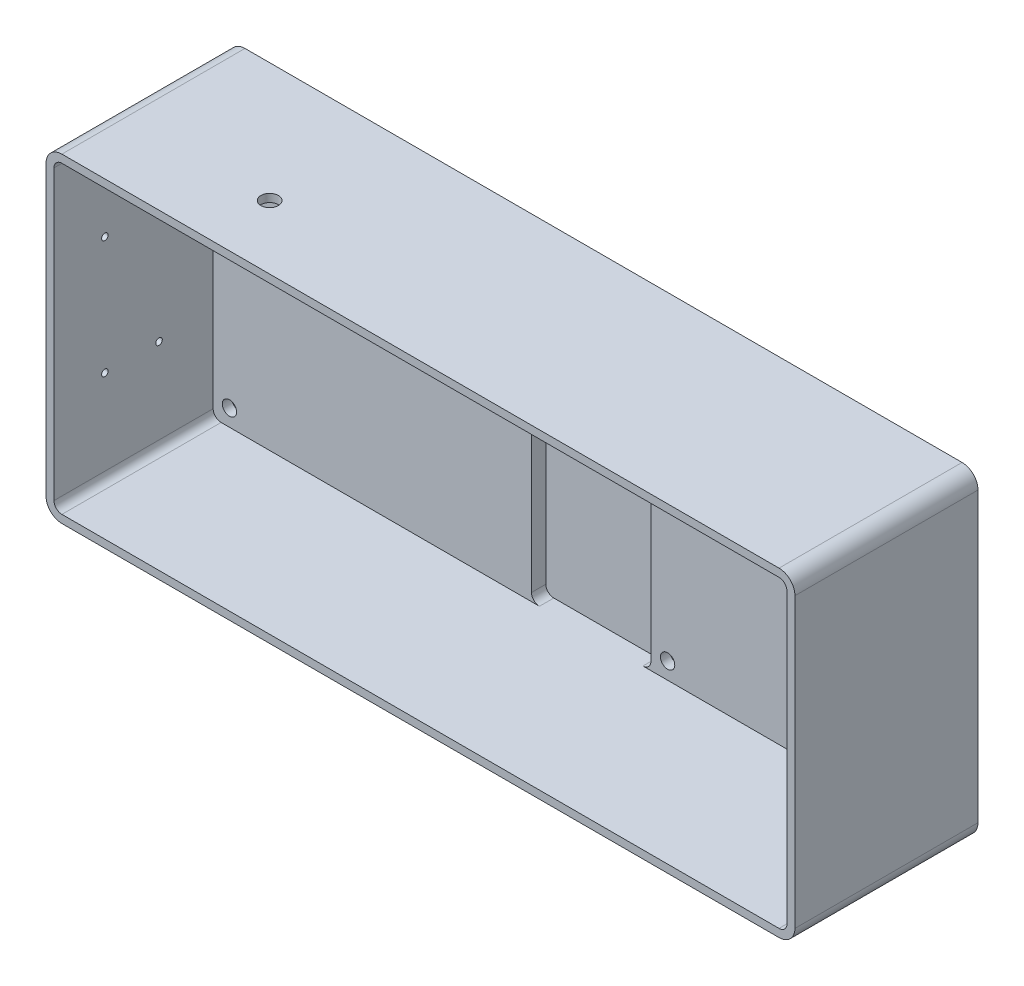
SolidWorks part; units mm, degrees
ref_plane "Front Plane" through (0, 0, 0) normal (0, 0, 1) x (1, 0, 0)
ref_plane "Top Plane" through (0, 0, 0) normal (0, 1, 0) x (1, 0, 0)
ref_plane "Right Plane" through (0, 0, 0) normal (1, 0, 0) x (0, 0, -1)
sketch "Sketch1" plane through (0, 0, 0) normal (0, 0, 1) x (1, 0, 0)
  line L0 (285.5, 0) -> (285.5, -100.5)
  line L1 (-185, 100.5) -> (185, 100.5)
  line L2 (-185, 100.5) -> (-185, -100.5)
  line L3 (-185, -100.5) -> (185, -100.5)
  line L5 (-185, 100.5) -> (185, -100.5) construction
  line L6 (-185, -100.5) -> (185, 100.5) construction
  line L7 (285.5, -100.5) -> (185, -100.5)
  line L8 (185, 100.5) -> (285.5, 100.5)
  line L9 (285.5, 100.5) -> (285.5, 0)
  point P0 (0, 0)
  dimension "D1" = 201
  dimension "D2" = 370
extrude "Boss-Extrude1" add sketch "Sketch1" along normal blind 115
shell "Shell1" thickness 5
sketch "Sketch5" plane through (-84.5, 100.5, 0) normal (0, 1, 0) x (0, 0, 1)
  line L1 (115, 370) -> (115, -100.5) construction
  line L2 (115, -100.5) -> (0, -100.5) construction
  circle A0 centre (75, 0) radius 5.5
  dimension "D1" = 11
  dimension "D3" = 40
  dimension "D4" = 100.5
extrude "Cut-Extrude4" cut sketch "Sketch5" against normal blind 10
sketch "Sketch6" plane through (-185, 0, 0) normal (-1, 0, 0) x (0, 0, 1)
  line L1 (83, 37) -> (49, 37)
  line L2 (83, 37) -> (83, -37) construction
  line L3 (83, -37) -> (49, -37) construction
  line L4 (49, 37) -> (49, -37) construction
  line L5 (83, 37) -> (49, -37) construction
  line L6 (83, -37) -> (49, 37) construction
  circle A0 centre (49, -37) radius 2.05
  circle A1 centre (49, 37) radius 2.05
  circle A2 centre (83, 37) radius 2.05
  circle A3 centre (83, -37) radius 2.05
  point P0 (66, 0)
  dimension "D4" = 4.1
  dimension "D1" = 66
  dimension "D2" = 74
  dimension "D3" = 34
extrude "Cut-Extrude5" cut sketch "Sketch6" against normal blind 10
fillet "Fillet1" radius 10 4 edges at (285.5, -100.5, 57.5) (285.5, 100.5, 57.5) (-185, 100.5, 57.5) (-185, -100.5, 57.5)
fillet "Fillet2" radius 5 4 edges at (280.5, 95.5, 60) (280.5, -95.5, 60) (-180, -95.5, 60) (-180, 95.5, 60)
sketch "Sketch7" plane through (0, 0, 5) normal (0, 0, 1) x (1, 0, 0)
  line L4 (280.5, -90.5) -> (280.5, 90.5)
  line L5 (275.5, 95.5) -> (-175, 95.5)
  line L6 (-180, 90.5) -> (-180, -90.5)
  line L7 (-175, -95.5) -> (275.5, -95.5)
  line L8 (280.5, -90.5) -> (280.5, 90.5)
  line L9 (275.5, 95.5) -> (-175, 95.5)
  line L10 (-180, 90.5) -> (-180, -90.5)
  line L11 (-175, -95.5) -> (275.5, -95.5)
  arc A4 (280.5, 90.5) -> (275.5, 95.5) centre (275.5, 90.5) ccw
  arc A5 (-175, 95.5) -> (-180, 90.5) centre (-175, 90.5) ccw
  arc A6 (-180, -90.5) -> (-175, -95.5) centre (-175, -90.5) ccw
  arc A7 (275.5, -95.5) -> (280.5, -90.5) centre (275.5, -90.5) ccw
  arc A8 (280.5, 90.5) -> (275.5, 95.5) centre (275.5, 90.5) ccw
  arc A9 (-175, 95.5) -> (-180, 90.5) centre (-175, 90.5) ccw
  arc A10 (-180, -90.5) -> (-175, -95.5) centre (-175, -90.5) ccw
  arc A11 (275.5, -95.5) -> (280.5, -90.5) centre (275.5, -90.5) ccw
  dimension "D1" = 0
extrude "Boss-Extrude2" add sketch "Sketch7" along normal blind 10
hole_wizard "Hole size per socket head cap screw type1" positions "Sketch8" profile "Sketch9" counterbore size "M8" standard "GB" end condition through all
sketch "Sketch8" plane through (0, 0, 0) normal (0, 0, -1) x (-1, 0, 0)
  line L0 (0, 0) -> (305.5658, 0) construction
  line L2 (-50.25, 100.5) -> (-50.25, 155.7325) construction
  line L3 (-275.5, 100.5) -> (175, 100.5) construction
  line L5 (-285.5, -90.5) -> (-285.5, 90.5) construction
  point P0 (-270.25, -85)
  point P2 (-270.25, 85)
  point P4 (169.75, 85)
  point P6 (169.75, -85)
  point P8 (-105.5, -85)
  point P10 (-105.5, 85)
  dimension "D1" = 440
  dimension "D2" = 170
  dimension "D3" = 180
  dimension "D4" = 170
sketch "Sketch9" plane through (270.25, -85, 0) normal (1, 0, 0) x (0, 1, 0)
  line L0 (0, 0) -> (0, 115)
  line L1 (0, 115) -> (4.5, 115)
  line L3 (4.5, 115) -> (4.5, 9)
  line L4 (4.5, 9) -> (7.5, 9)
  line L5 (7.5, 9) -> (7.5, 0)
  line L7 (7.5, 0) -> (0, 0)
  line L11 (0, -6.35) -> (0, 107.95) construction
  dimension "通孔孔直径" = 9
  dimension "通孔孔深度" = 115
  dimension "柱形沉头孔直径" = 15
  dimension "柱形沉头孔深度" = 9
sketch "Sketch10" plane through (0, 0, 15) normal (0, 0, 1) x (1, 0, 0)
  line L0 (285.5, -90.5) -> (285.5, 90.5) construction
  line L1 (95, 95.5) -> (20, 95.5)
  line L2 (95, 95.5) -> (95, -95.5)
  line L3 (95, -95.5) -> (20, -95.5)
  line L4 (20, 95.5) -> (20, -95.5)
  line L5 (95, 95.5) -> (20, -95.5) construction
  line L6 (95, -95.5) -> (20, 95.5) construction
  line L7 (0, 0) -> (134.369, 0) construction
  point P0 (57.5, 0)
  dimension "D1" = 191
  dimension "D2" = 75
  dimension "D3" = 190.5
extrude "Cut-Extrude6" cut sketch "Sketch10" against normal blind 9
fillet "Fillet3" radius 5 4 edges at (95, 95.5, 10.5) (20, 95.5, 10.5) (20, -95.5, 10.5) (95, -95.5, 10.5)
